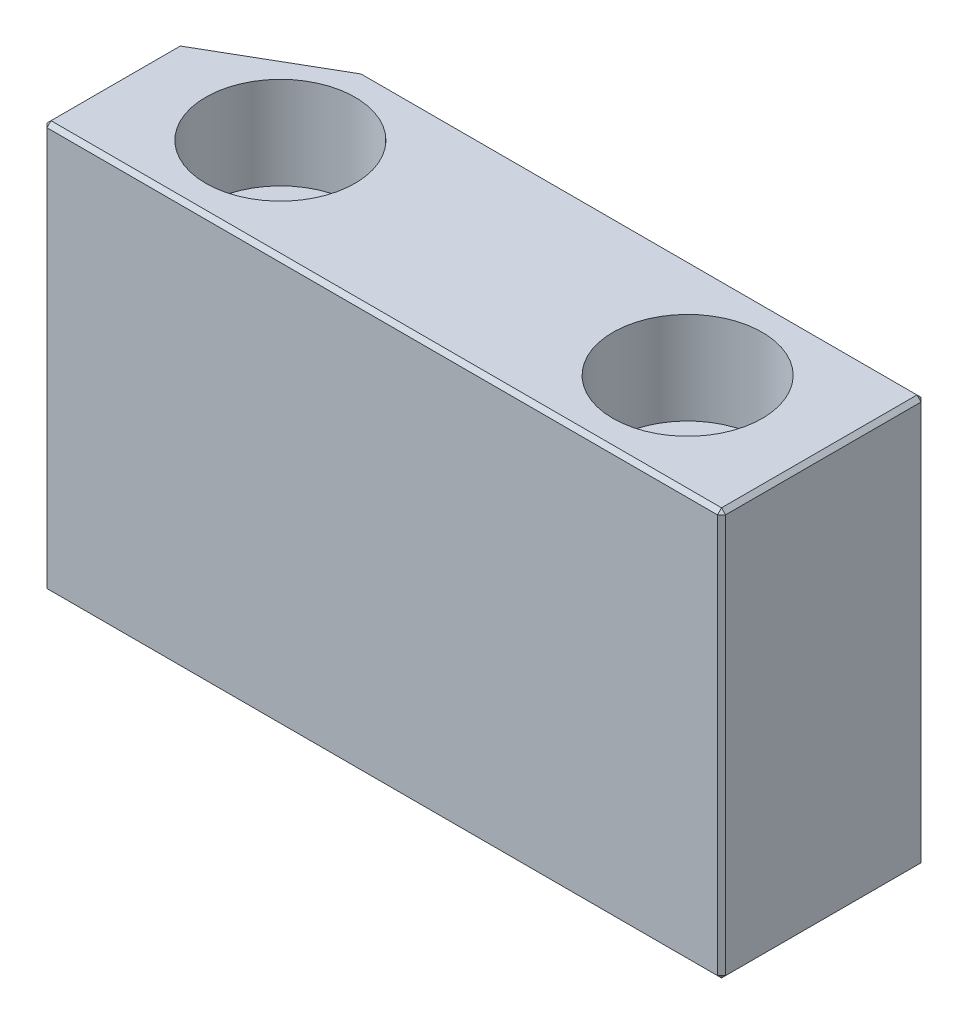
from build123d import *

# Parameters (mm, degrees)
SKETCH_1_W                = 50
SKETCH_1_H                = 30
EXTRUDE_1_DEPTH           = 15
HOLE_WIZARD_1_D           = 6.6
HOLE_WIZARD_1_CBORE_D     = 11
HOLE_WIZARD_1_CBORE_DEPTH = 6.8
CHAMFER_1_SIZE            = 5
CHAMFER_1_SIZE2           = 8.660254038
CHAMFER_2_SIZE            = 0.3


with BuildPart() as part:
    # 草图1 → 凸台-拉伸1 (new body)
    with BuildSketch(Plane.XY):
        Rectangle(SKETCH_1_W, SKETCH_1_H)
    extrude(amount=EXTRUDE_1_DEPTH)

    # 打孔尺寸根据内六角圆柱头螺钉的类型1 (through all)
    with Locations(Plane(origin=(0, 15, 0), x_dir=(1, 0, 0), z_dir=(0, 1, 0))):
        with Locations((-15, -7.5), (15, -7.5)):
            CounterBoreHole(HOLE_WIZARD_1_D / 2, HOLE_WIZARD_1_CBORE_D / 2, HOLE_WIZARD_1_CBORE_DEPTH)

    # 倒角1
    chamfer_1_edges = [part.edges().sort_by_distance(p)[0] for p in [
        (-25, 0, 0),
    ]]
    chamfer_1_side = [part.faces().sort_by_distance(p)[0] for p in [
        (-25, 0, 7.5),
    ]]
    chamfer(chamfer_1_edges, length=CHAMFER_1_SIZE, length2=CHAMFER_1_SIZE2, reference=chamfer_1_side[0])

    # 倒角2
    chamfer_2_edges = [part.edges().sort_by_distance(p)[0] for p in [
        (-25, 0, 15),
        (0, -15, 15),
        (4.330127019, -15, 0),
        (-20.669872981, -15, 2.5),
        (-20.669872981, 15, 2.5),
        (25, 0, 15),
        (4.330127019, 15, 0),
        (25, 0, 0),
        (0, 15, 15),
        (25, -15, 7.5),
        (-25, -15, 10),
        (-25, 15, 10),
        (25, 15, 7.5),
    ]]
    chamfer(chamfer_2_edges, length=CHAMFER_2_SIZE)


solid = part.part
